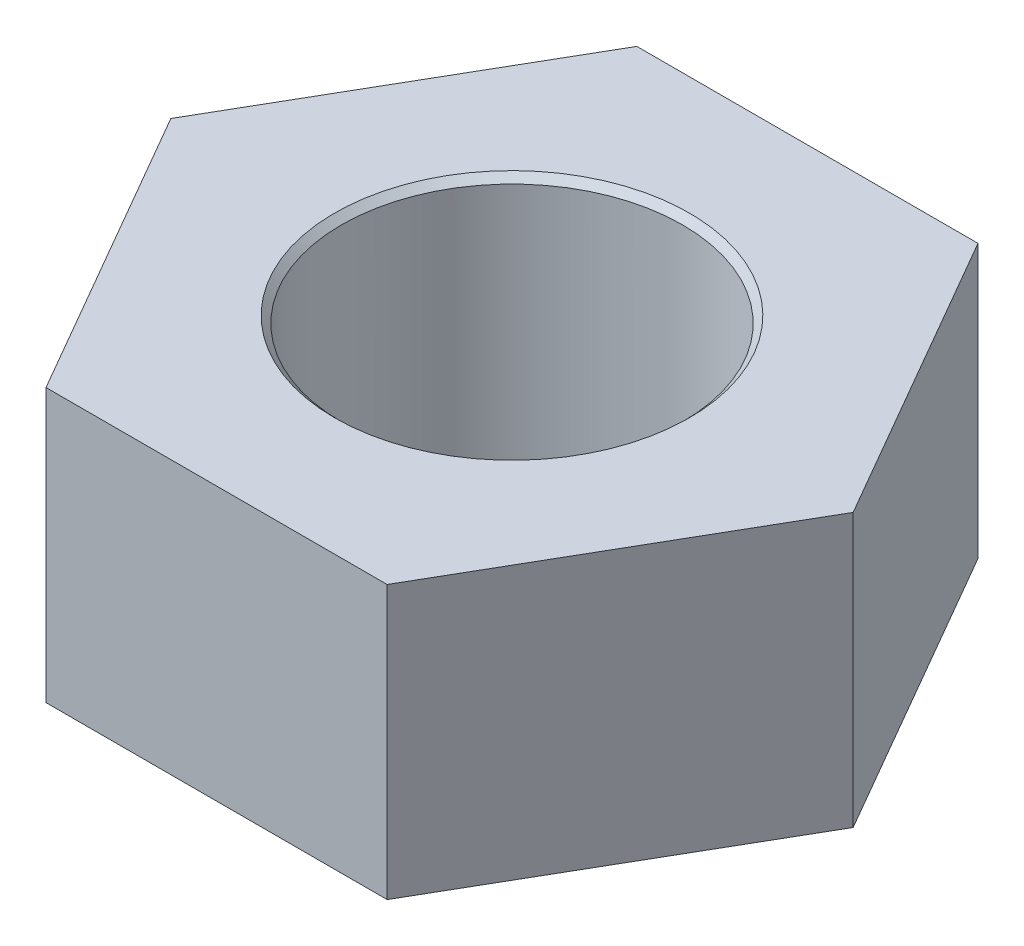
from build123d import *

# Parameters (mm, degrees)
SKETCH1_R           = 2.5
BOSS_EXTRUDE1_DEPTH = 4
CHAMFER1_SIZE       = 0.1


with BuildPart() as part:
    # Sketch1 → Boss-Extrude1 (new body)
    with BuildSketch(Plane(origin=(0, 0, 0), x_dir=(1, 0, 0), z_dir=(0, 1, 0))):
        Polygon((2.5, -4.330127019), (5, 0), (2.5, 4.330127019), (-2.5, 4.330127019), (-5, 0), (-2.5, -4.330127019), align=None)
        with Locations(Location((0, 0, 0), (0, 0, 270))):
            Circle(SKETCH1_R, mode=Mode.SUBTRACT)
    extrude(amount=BOSS_EXTRUDE1_DEPTH)

    # Chamfer1
    chamfer1_edges = [part.edges().sort_by_distance(p)[0] for p in [
        (0, 0, -2.5),
        (0, 4, -2.5),
    ]]
    chamfer(chamfer1_edges, length=CHAMFER1_SIZE)


solid = part.part
